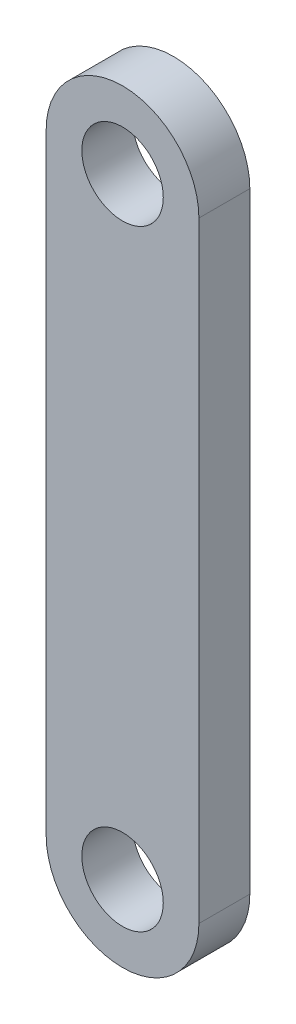
SolidWorks part; units mm, degrees
ref_plane "Front Plane" through (0, 0, 0) normal (0, 0, 1) x (1, 0, 0)
ref_plane "Top Plane" through (0, 0, 0) normal (0, 1, 0) x (1, 0, 0)
ref_plane "Right Plane" through (0, 0, 0) normal (1, 0, 0) x (0, 0, -1)
other "Configuration Table"
sketch "Sketch1" plane through (0, 0, 0) normal (0, 0, 1) x (1, 0, 0)
  line L0 (0, 75) -> (0, -45) construction
  line L2 (-15, 60) -> (-15, -60)
  line L4 (15, 60) -> (15, -60)
  line L5 (-15, 75) -> (0, 0) construction
  line L6 (-13.3629, -66.8143) -> (-9.7141, -48.5704) construction
  line L7 (0, 0) -> (15, 75) construction
  line L8 (0, -52) -> (0, -75) construction
  line L9 (9.7141, -48.5704) -> (13.3629, -66.8143) construction
  circle A0 centre (0, 60) radius 8
  circle A1 centre (0, -60) radius 8
  arc A2 (15, 60) -> (-15, 60) centre (0, 60) ccw
  arc A3 (-15, -60) -> (15, -60) centre (0, -60) ccw
  point P0 (0, 0)
  dimension "D1" = 120
  dimension "D2" = 16
  dimension "D3" = 30
extrude "Boss-Extrude1" add sketch "Sketch1" along normal blind 10
